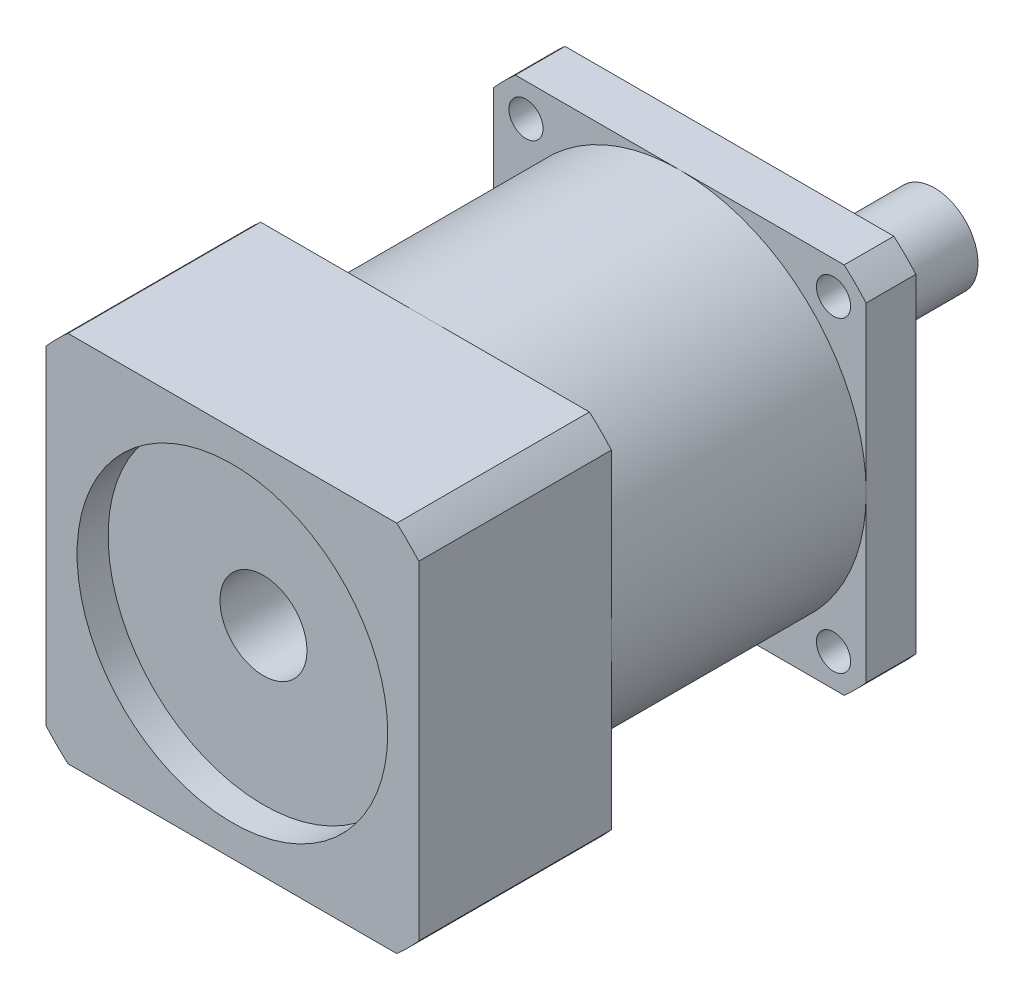
SolidWorks part; units mm, degrees
ref_plane "前视基准面" through (0, 0, 0) normal (0, 0, 1) x (1, 0, 0)
ref_plane "上视基准面" through (0, 0, 0) normal (0, 1, 0) x (1, 0, 0)
ref_plane "右视基准面" through (0, 0, 0) normal (1, 0, 0) x (0, 0, -1)
sketch "草图1" plane through (0, 0, 0) normal (0, 0, 1) x (1, 0, 0)
  circle A0 centre (0, 0) radius 7
  dimension "D1" = 14
extrude "凸台-拉伸1" add sketch "草图1" along normal blind 30
sketch "草图2" plane through (0, 0, 30) normal (0, 0, 1) x (1, 0, 0)
  circle A0 centre (0, 0) radius 25
  dimension "D1" = 50
extrude "凸台-拉伸2" add sketch "草图2" along normal blind 3
sketch "草图3" plane through (0, 0, 33) normal (0, 0, 1) x (1, 0, 0)
  line L1 (-30, 30) -> (30, 30)
  line L2 (-30, 30) -> (-30, -30)
  line L3 (-30, -30) -> (30, -30)
  line L4 (30, 30) -> (30, -30)
  line L5 (-30, 30) -> (30, -30) construction
  line L6 (-30, -30) -> (30, 30) construction
  point P0 (0, 0)
  dimension "D1" = 60
  dimension "D2" = 60
extrude "凸台-拉伸3" add sketch "草图3" along normal blind 8
sketch "草图4" plane through (0, 0, 41) normal (0, 0, 1) x (1, 0, 0)
  circle A0 centre (0, 0) radius 30
  dimension "D1" = 60
extrude "凸台-拉伸4" add sketch "草图4" along normal blind 41
sketch "草图5" plane through (0, 0, 82) normal (0, 0, 1) x (1, 0, 0)
  line L1 (-30, 30) -> (30, 30)
  line L2 (-30, 30) -> (-30, -30)
  line L3 (-30, -30) -> (30, -30)
  line L4 (30, 30) -> (30, -30)
  line L5 (-30, 30) -> (30, -30) construction
  line L6 (-30, -30) -> (30, 30) construction
  point P0 (0, 0)
  dimension "D1" = 60
  dimension "D2" = 60
extrude "凸台-拉伸5" add sketch "草图5" along normal blind 31
ref_axis "基准轴1" through (0, 0, 82) along (0, 0, -1)
sketch "草图6" plane through (0, 0, 0) normal (0, 1, 0) x (1, 0, 0)
  line L0 (30, -113) -> (-30, -113) construction
  line L1 (-47.3403, -33) -> (-40, -33)
  line L2 (-47.3403, -33) -> (-47.3403, -113)
  line L3 (-47.3403, -113) -> (-40, -113)
  line L4 (-40, -33) -> (-40, -113)
  line L5 (30, -33) -> (-30, -33) construction
  line L6 (0, -82) -> (0, -41) construction
  dimension "D1" = 40
revolve "切除-旋转1" cut sketch "草图6" angle 360 about axis through (0, 0, 82) along (0, 0, -1)
sketch "草图7" plane through (0, 0, 33) normal (0, 0, -1) x (-1, 0, 0)
  line L0 (0, 0) -> (30, 0) construction
  line L1 (0, 0) -> (0, 30) construction
  line L2 (-26.4575, 30) -> (26.4575, 30) construction
  line L3 (0, 0) -> (28.2843, 28.2843) construction
  circle A0 centre (-24.7487, 24.7487) radius 2.75
  arc A1 (30, 26.4575) -> (26.4575, 30) centre (0, 0) ccw construction
  circle A2 centre (24.7487, 24.7487) radius 2.75
  circle A3 centre (-24.7487, -24.7487) radius 2.75
  circle A4 centre (24.7487, -24.7487) radius 2.75
  dimension "D1" = 5.5
  dimension "D2" = 70
extrude "切除-拉伸1" cut sketch "草图7" against normal up to next
sketch "草图8" plane through (0, 0, 113) normal (0, 0, 1) x (1, 0, 0)
  circle A0 centre (0, 0) radius 25
  dimension "D1" = 50
extrude "切除-拉伸2" cut sketch "草图8" against normal blind 5
sketch "草图9" plane through (0, 0, 108) normal (0, 0, 1) x (1, 0, 0)
  circle A0 centre (0, 0) radius 7
  dimension "D1" = 14
extrude "切除-拉伸3" cut sketch "草图9" against normal blind 25
